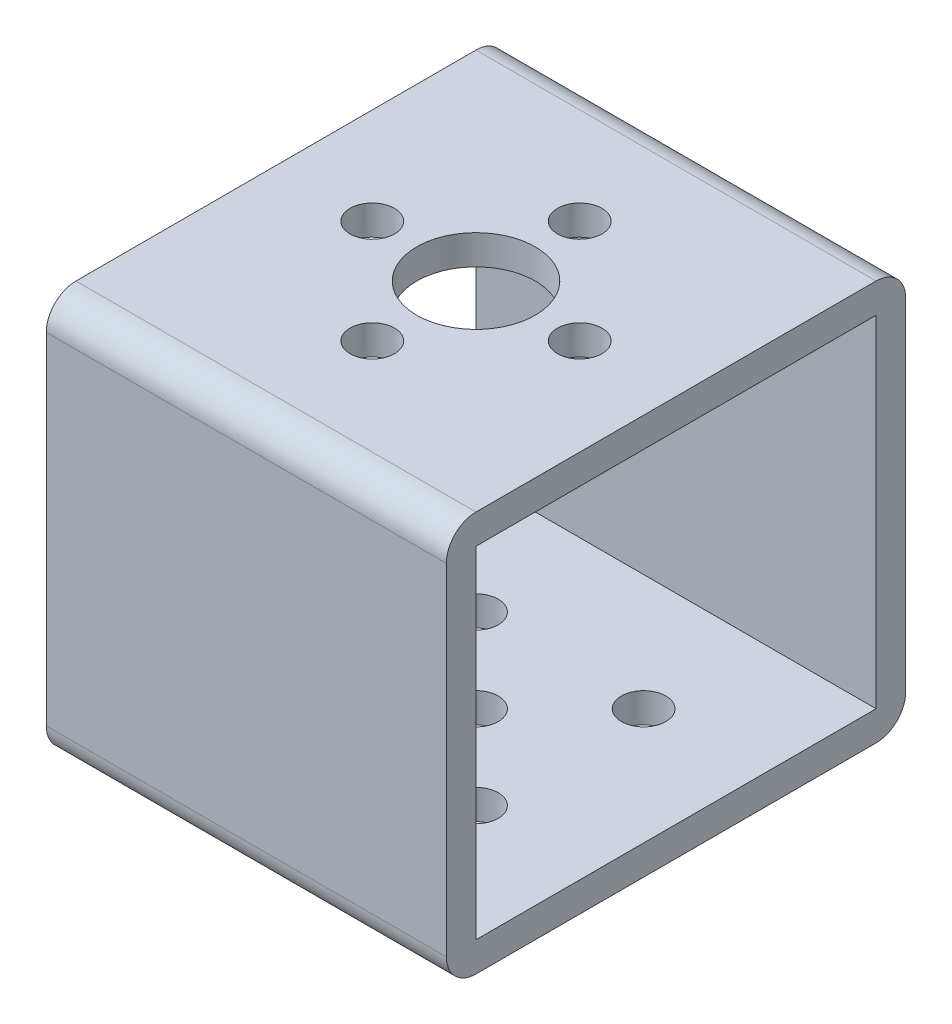
SolidWorks part; units mm, degrees
ref_plane "Front Plane" through (0, 0, 0) normal (0, 0, 1) x (1, 0, 0)
ref_plane "Top Plane" through (0, 0, 0) normal (0, 1, 0) x (1, 0, 0)
ref_plane "Right Plane" through (0, 0, 0) normal (1, 0, 0) x (0, 0, -1)
other "Configuration Table"
sketch "Sketch1" plane through (0, 0, 0) normal (0, 0, 1) x (1, 0, 0)
  line L1 (-13.5, 13.5) -> (13.5, 13.5)
  line L2 (-13.5, 13.5) -> (-13.5, -13.5)
  line L3 (-13.5, -13.5) -> (13.5, -13.5)
  line L4 (13.5, 13.5) -> (13.5, -13.5)
  line L5 (-13.5, 13.5) -> (13.5, -13.5) construction
  line L6 (-13.5, -13.5) -> (13.5, 13.5) construction
  point P0 (0, 0)
  dimension "D1" = 27
  dimension "27" = 27
extrude "Boss-Extrude1" add sketch "Sketch1" along normal blind 29
sketch "Sketch2" plane through (13.5, 0, 0) normal (1, 0, 0) x (0, 0, -1)
  line L0 (-29, -13.5) -> (-29, 13.5) construction
  line L1 (-29, 11.5) -> (-2, 11.5)
  line L2 (-29, 11.5) -> (-29, -11.5)
  line L3 (-29, -11.5) -> (-2, -11.5)
  line L4 (-2, 11.5) -> (-2, -11.5)
  line L5 (-29, 13.5) -> (0, 13.5) construction
  line L6 (-29, -13.5) -> (0, -13.5) construction
  line L7 (0, -13.5) -> (0, 13.5) construction
  dimension "D1" = 2
  dimension "D2" = 2
  dimension "D3" = 2
extrude "Cut-Extrude1" cut sketch "Sketch2" against normal blind 27
sketch "Sketch4" plane through (0, 13.5, 0) normal (0, 1, 0) x (1, 0, 0)
  line L0 (0, 0) -> (0, -30.566) construction
  line L2 (13.5, -29) -> (-13.5, -29) construction
  line L3 (0, -15.5) -> (28.6851, -15.5) construction
  circle A0 centre (0, -15.5) radius 4
  circle A1 centre (0, -15.5) radius 7 construction
  circle A2 centre (0, -8.5) radius 1.5
  circle A3 centre (7, -15.5) radius 1.5
  circle A4 centre (0, -22.5) radius 1.5
  circle A5 centre (-7, -15.5) radius 1.5
  point P19 (0, -15.5)
  dimension "D1" = 8
  dimension "D2" = 3
  dimension "D3" = 14
  dimension "D4" = 13.5
  dimension "D5" = 4
extrude "Cut-Extrude2" cut sketch "Sketch4" against normal up to next
sketch "Sketch5" plane through (0, -13.5, 0) normal (0, -1, 0) x (1, 0, 0)
  line L0 (0, 0) -> (0, 30.8311) construction
  line L1 (-13.5, 0) -> (13.5, 0) construction
  line L2 (-13.5, 29) -> (13.5, 29) construction
  line L3 (0, 15.5) -> (-10.8732, 26.3732) construction
  line L4 (0, 15.5) -> (11.3033, 26.8033) construction
  circle A0 centre (0, 15.5) radius 1.5
  circle A1 centre (0, 15.5) radius 8 construction
  circle A8 centre (-5.6569, 21.1569) radius 1.5
  circle A9 centre (5.6569, 21.1569) radius 1.5
  circle A10 centre (5.6569, 9.8431) radius 1.5
  circle A11 centre (-5.6569, 9.8431) radius 1.5
  point P20 (0, 15.5)
  point P27 (0, 15.5)
  dimension "D1" = 3
  dimension "D3" = 16
  dimension "D6" = 3
  dimension "D4" = 13.5
  dimension "D5" = 45
  dimension "D7" = 4
extrude "Cut-Extrude3" cut sketch "Sketch5" against normal up to next
fillet "Fillet1" radius 2 2 edges at (0, 13.5, 0) (0, -13.5, 0)
sketch "Sketch6" plane through (0, -13.5, 0) normal (0, -1, 0) x (1, 0, 0)
  line L1 (-13.5, 29) -> (13.5, 29)
  line L2 (-13.5, 29) -> (-13.5, 31)
  line L3 (-13.5, 31) -> (13.5, 31)
  line L4 (13.5, 29) -> (13.5, 31)
  dimension "D1" = 2
  dimension "D2" = 27
extrude "Boss-Extrude2" add sketch "Sketch6" against normal up to surface (27 mm away) up to face at (0, 13.5, 10)
fillet "Fillet2" radius 2 2 edges at (0, 13.5, 31) (0, -13.5, 31)
